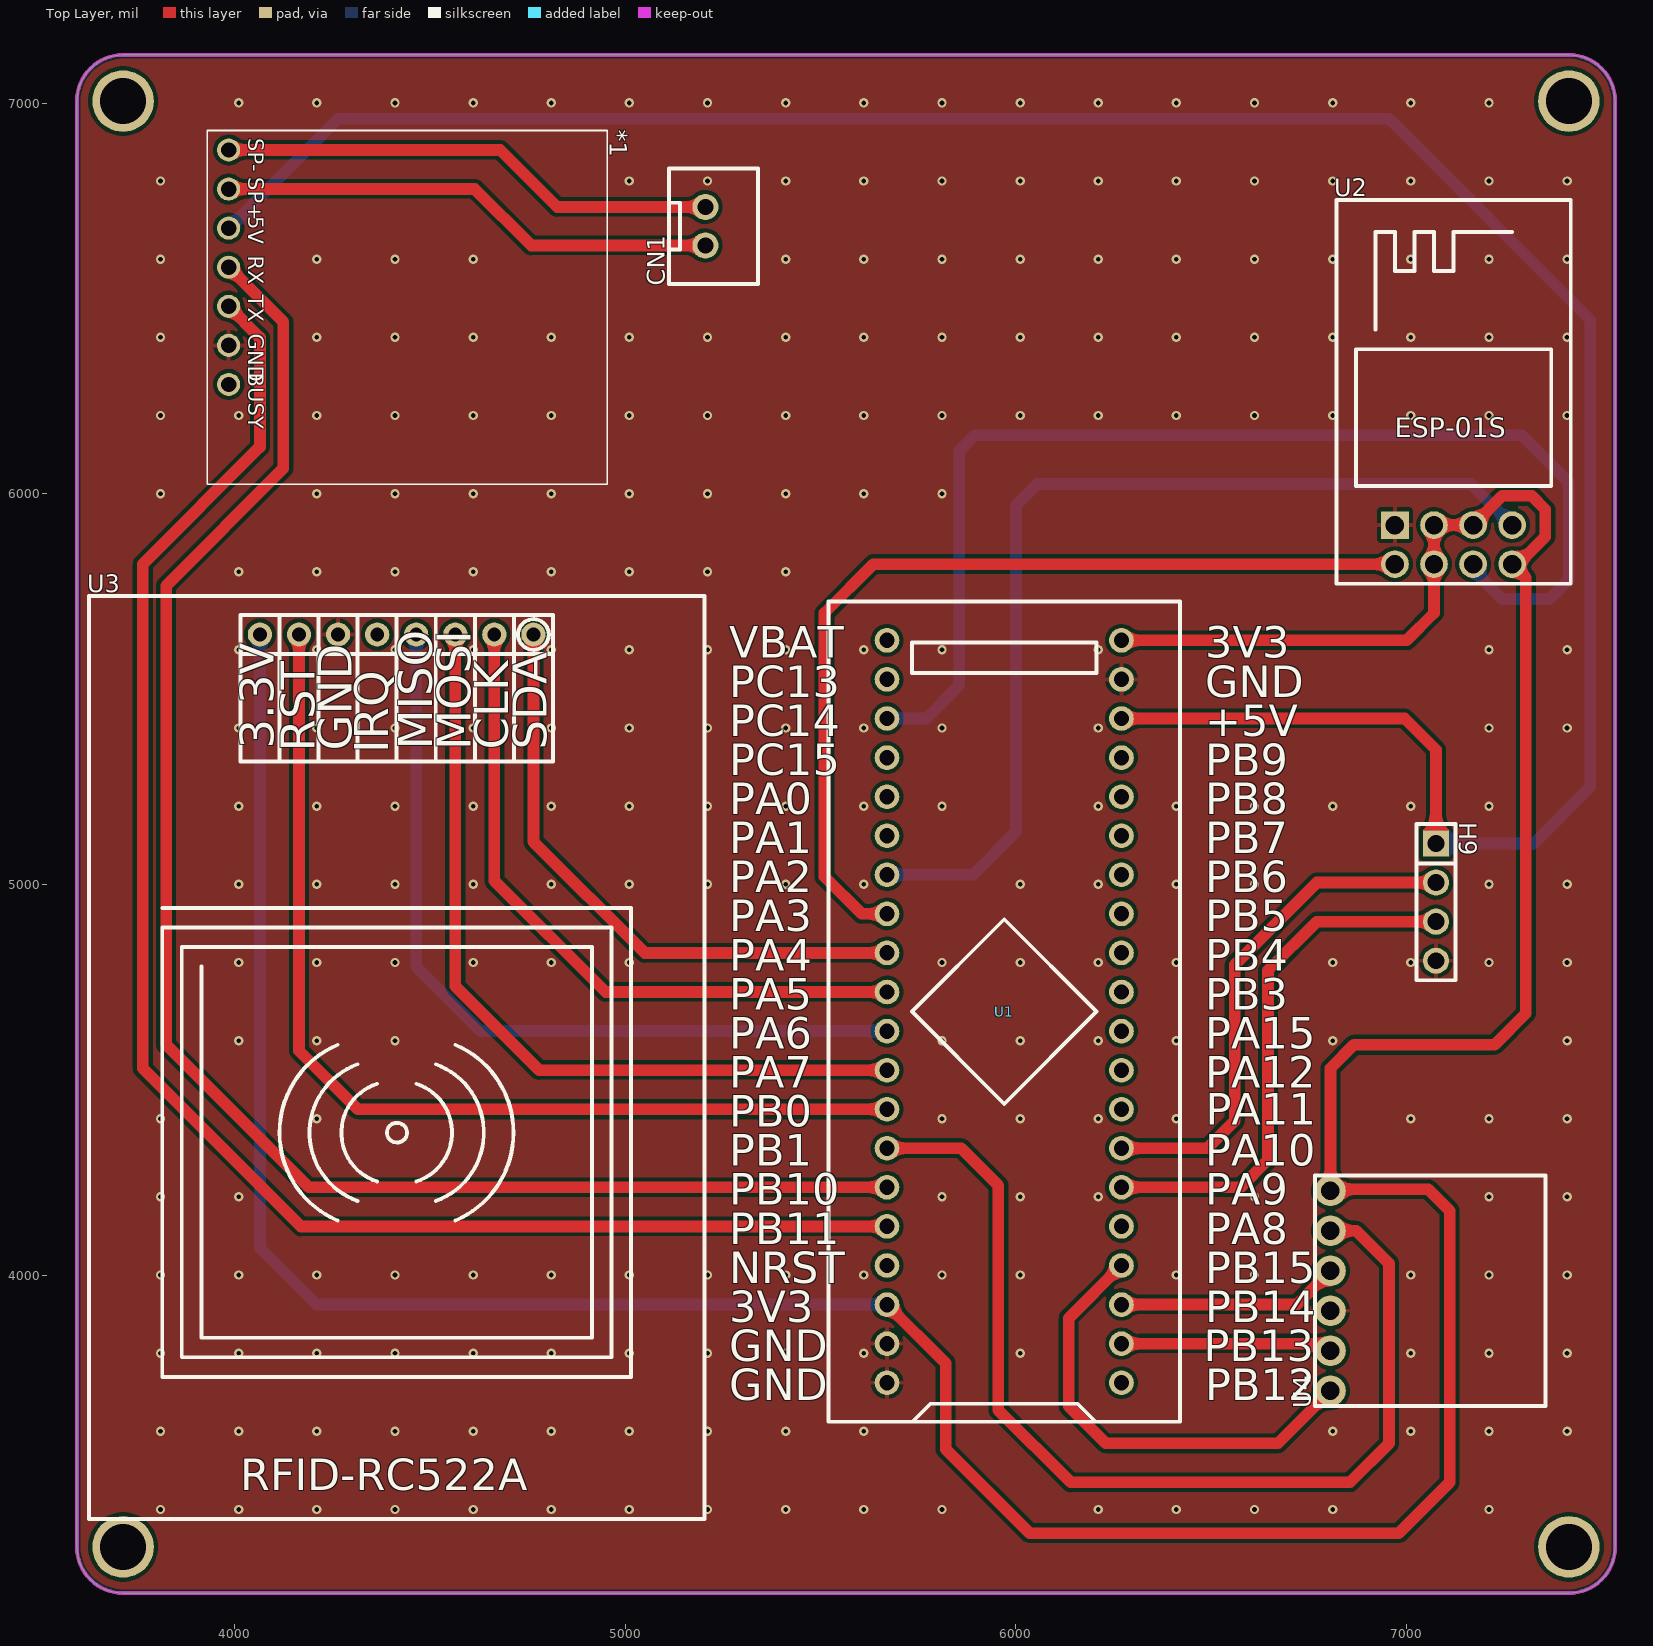
[diagram p0: Top Layer view]
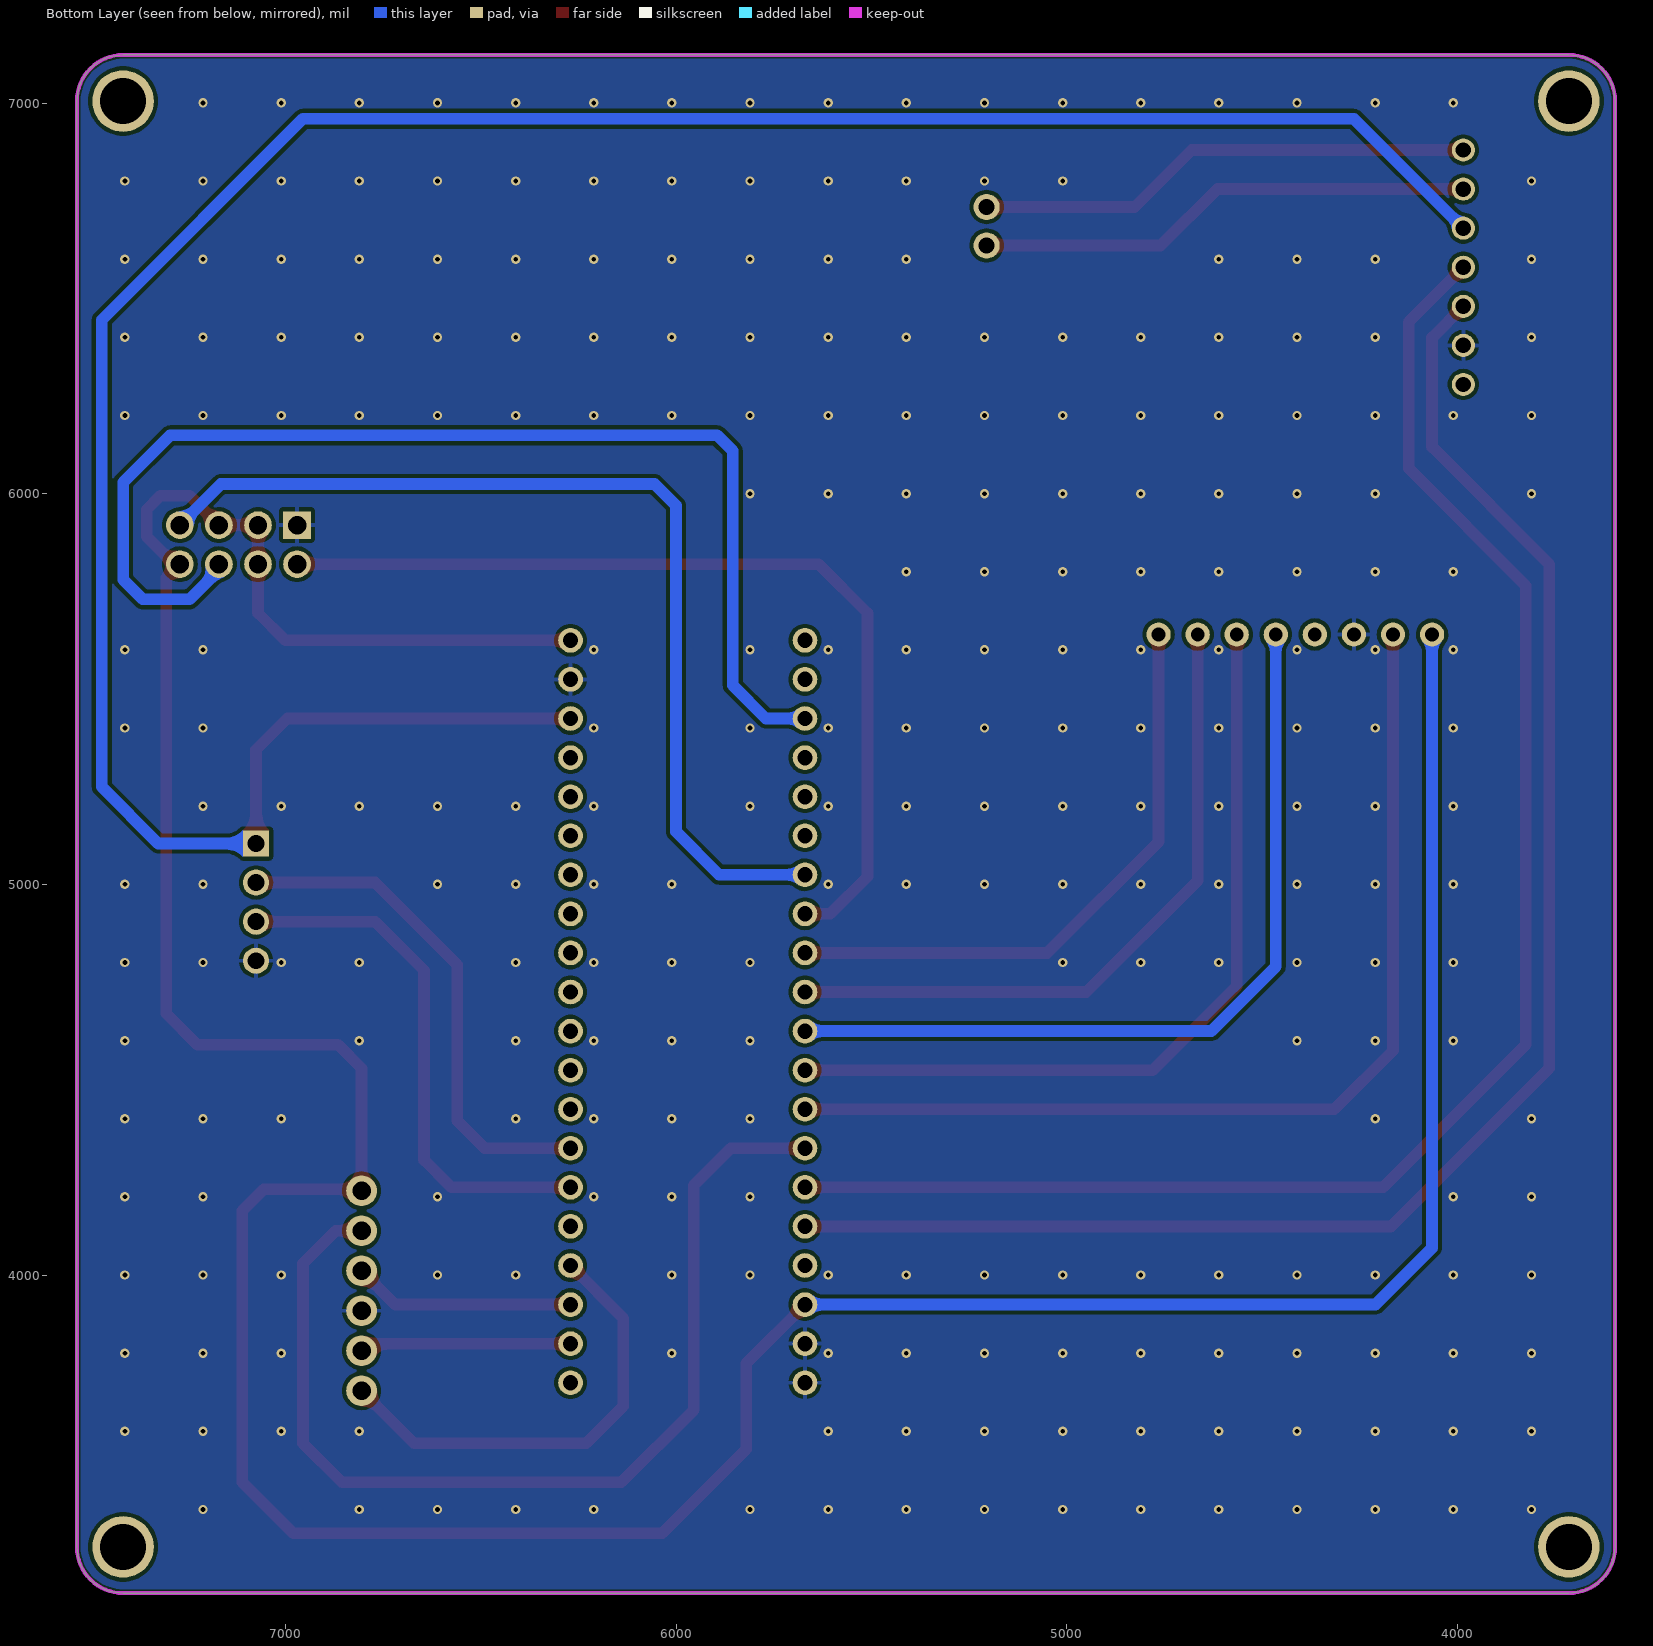
[diagram p1: Bottom Layer view, seen from below]
# Altium PCB MISC51107.pcbdoc
Units mil, origin at the board's own origin, x right, y up, seen from the top; angles counter-clockwise.
Board outline 3937.01 x 3937.01 mil, 2 copper layers (Top Layer, Bottom Layer), stack 62.206 mil thick; 7 components, 39 nets, 79 pads, 259 vias.

## Layer stack, top to bottom
Top Solder Mask Layer: solder mask 0.394, Dk 3.3
Top Layer: signal copper 1.379
Dielectric1: surface 59.449, FR4, Dk 4.5
Bottom Layer: signal copper 1.378
Bottom Solder Mask Layer: solder mask 0.394, Dk 3.3

## Board outline
3714.61,7123.5 ccw(c3714.61,7005.39) 3596.5,7005.39 3596.5,3304.61 ccw(c3714.61,3304.61) 3714.61,3186.5 7415.39,3186.5 ccw(c7415.39,3304.61) 7533.5,3304.61 7533.5,7005.39 ccw(c7415.39,7005.39) 7415.39,7123.5 3714.61,7123.5

## Design rules (kind name [scope] priority, off if disabled: settings)
BoardOutlineClearance copperThickness2oz_1 [All] p2 off: genericclearance=7.99 ignorepadtopadclearanceinfootprint=FALSE except(0: Arc-SplitContinuation Track-SplitContinuation SMDPad-SplitContinuation THPad-SplitContinuation Via-SplitContinuation Fill-SplitContinuation Region-SplitContinuation Poly-SplitContinuation Text-SplitContinuation Hole-SplitContinuation; 5.98: Arc-CutoutEdge Track-CutoutEdge SMDPad-CutoutEdge THPad-CutoutEdge Via-CutoutEdge Text-CutoutEdge; 6.9: Hole-OutlineEdge Hole-CutoutEdge; 10: Poly-OutlineEdge Poly-CutoutEdge; 11.81: Arc-OutlineEdge Track-OutlineEdge SMDPad-OutlineEdge THPad-OutlineEdge Via-OutlineEdge Fill-OutlineEdge Region-OutlineEdge Text-OutlineEdge Fill-CutoutEdge Region-CutoutEdge)
BoardOutlineClearance Plane_innerPlane_1 [All] p4 off: genericclearance=4.02 ignorepadtopadclearanceinfootprint=FALSE except(0: Arc-SplitContinuation Track-SplitContinuation SMDPad-SplitContinuation THPad-SplitContinuation Via-SplitContinuation Fill-SplitContinuation Region-SplitContinuation Poly-SplitContinuation Text-SplitContinuation Hole-SplitContinuation; 5.98: Arc-CutoutEdge Track-CutoutEdge SMDPad-CutoutEdge THPad-CutoutEdge Via-CutoutEdge Text-CutoutEdge; 6.9: Hole-OutlineEdge Hole-CutoutEdge; 10: Poly-OutlineEdge Poly-CutoutEdge; 11.81: Arc-OutlineEdge Track-OutlineEdge SMDPad-OutlineEdge THPad-OutlineEdge Via-OutlineEdge Fill-OutlineEdge Region-OutlineEdge Text-OutlineEdge Fill-CutoutEdge Region-CutoutEdge)
BoardOutlineClearance Copper_copperRegion_1 [All] p6 off: genericclearance=4.02 ignorepadtopadclearanceinfootprint=FALSE except(0: Arc-SplitContinuation Track-SplitContinuation SMDPad-SplitContinuation THPad-SplitContinuation Via-SplitContinuation Fill-SplitContinuation Region-SplitContinuation Poly-SplitContinuation Text-SplitContinuation Hole-SplitContinuation; 5.98: Arc-CutoutEdge Track-CutoutEdge SMDPad-CutoutEdge THPad-CutoutEdge Via-CutoutEdge Text-CutoutEdge; 6.9: Hole-OutlineEdge Hole-CutoutEdge; 10: Poly-OutlineEdge Poly-CutoutEdge; 11.81: Arc-OutlineEdge Track-OutlineEdge SMDPad-OutlineEdge THPad-OutlineEdge Via-OutlineEdge Fill-OutlineEdge Region-OutlineEdge Text-OutlineEdge Fill-CutoutEdge Region-CutoutEdge)
BoardOutlineClearance Copper_copperRegion_copperThickness1oz_1 [All] p8 off: genericclearance=4.02 ignorepadtopadclearanceinfootprint=FALSE except(0: Arc-SplitContinuation Track-SplitContinuation SMDPad-SplitContinuation THPad-SplitContinuation Via-SplitContinuation Fill-SplitContinuation Region-SplitContinuation Poly-SplitContinuation Text-SplitContinuation Hole-SplitContinuation; 5.98: Arc-CutoutEdge Track-CutoutEdge SMDPad-CutoutEdge THPad-CutoutEdge Via-CutoutEdge Text-CutoutEdge; 6.9: Hole-OutlineEdge Hole-CutoutEdge; 10: Poly-OutlineEdge Poly-CutoutEdge; 11.81: Arc-OutlineEdge Track-OutlineEdge SMDPad-OutlineEdge THPad-OutlineEdge Via-OutlineEdge Fill-OutlineEdge Region-OutlineEdge Text-OutlineEdge Fill-CutoutEdge Region-CutoutEdge)
BoardOutlineClearance Copper_copperRegion_Copper_copperRegion_1 [All] p10 off: genericclearance=4.02 ignorepadtopadclearanceinfootprint=FALSE except(0: Arc-SplitContinuation Track-SplitContinuation SMDPad-SplitContinuation THPad-SplitContinuation Via-SplitContinuation Fill-SplitContinuation Region-SplitContinuation Poly-SplitContinuation Text-SplitContinuation Hole-SplitContinuation; 5.98: Arc-CutoutEdge Track-CutoutEdge SMDPad-CutoutEdge THPad-CutoutEdge Via-CutoutEdge Text-CutoutEdge; 6.9: Hole-OutlineEdge Hole-CutoutEdge; 10: Poly-OutlineEdge Poly-CutoutEdge; 11.81: Arc-OutlineEdge Track-OutlineEdge SMDPad-OutlineEdge THPad-OutlineEdge Via-OutlineEdge Fill-OutlineEdge Region-OutlineEdge Text-OutlineEdge Fill-CutoutEdge Region-CutoutEdge)
BoardOutlineClearance copperThickness1oz_1 [All] p12: genericclearance=4.02 ignorepadtopadclearanceinfootprint=FALSE except(0: Arc-SplitContinuation Track-SplitContinuation SMDPad-SplitContinuation THPad-SplitContinuation Via-SplitContinuation Fill-SplitContinuation Region-SplitContinuation Poly-SplitContinuation Text-SplitContinuation Hole-SplitContinuation; 5.98: Arc-CutoutEdge Track-CutoutEdge SMDPad-CutoutEdge THPad-CutoutEdge Via-CutoutEdge Text-CutoutEdge; 6.9: Hole-OutlineEdge Hole-CutoutEdge; 10: Poly-OutlineEdge Poly-CutoutEdge; 11.81: Arc-OutlineEdge Track-OutlineEdge SMDPad-OutlineEdge THPad-OutlineEdge Via-OutlineEdge Fill-OutlineEdge Region-OutlineEdge Text-OutlineEdge Fill-CutoutEdge Region-CutoutEdge)
Clearance copperThickness2oz [All] p1 off: gap=7.99 ignorepadtopadclearanceinfootprint=FALSE except(5.98: SMDPad-Track SMDPad-SMDPad THPad-Track SMDPad-THPad THPad-THPad Track-Via SMDPad-Via THPad-Via Via-Via Fill-SMDPad Region-SMDPad Fill-THPad Region-THPad Fill-Via Region-Via Fill-Fill Fill-Region Region-Region Arc-Track Arc-SMDPad Arc-THPad Arc-Via Fill-Arc Region-Arc Arc-Arc Text-Track SMDPad-Text Text-THPad Text-Via Fill-Text Region-Text Arc-Text Text-Text; 6.9: Hole-Track Hole-SMDPad Hole-THPad Hole-Via Fill-Hole Region-Hole Hole-Arc Hole-Text; 10: Poly-Track Poly-SMDPad Poly-THPad Poly-Via Poly-Fill Poly-Region Poly-Poly Poly-Arc Poly-Text Poly-Hole; 11.81: Fill-Track Region-Track)
Clearance Plane_innerPlane [All] p3 off: gap=4.02 ignorepadtopadclearanceinfootprint=FALSE except(5.98: SMDPad-Track SMDPad-SMDPad THPad-Track SMDPad-THPad THPad-THPad Track-Via SMDPad-Via THPad-Via Via-Via Fill-SMDPad Region-SMDPad Fill-THPad Region-THPad Fill-Via Region-Via Fill-Fill Fill-Region Region-Region Arc-Track Arc-SMDPad Arc-THPad Arc-Via Fill-Arc Region-Arc Arc-Arc Text-Track SMDPad-Text Text-THPad Text-Via Fill-Text Region-Text Arc-Text Text-Text; 6.9: Hole-Track Hole-SMDPad Hole-THPad Hole-Via Fill-Hole Region-Hole Hole-Arc Hole-Text; 10: Poly-Track Poly-SMDPad Poly-THPad Poly-Via Poly-Fill Poly-Region Poly-Poly Poly-Arc Poly-Text Poly-Hole; 11.81: Fill-Track Region-Track)
Clearance Copper_copperRegion [All] p5 off: gap=4.02 ignorepadtopadclearanceinfootprint=FALSE except(5.98: SMDPad-Track SMDPad-SMDPad THPad-Track SMDPad-THPad THPad-THPad Track-Via SMDPad-Via THPad-Via Via-Via Fill-SMDPad Region-SMDPad Fill-THPad Region-THPad Fill-Via Region-Via Fill-Fill Fill-Region Region-Region Arc-Track Arc-SMDPad Arc-THPad Arc-Via Fill-Arc Region-Arc Arc-Arc Text-Track SMDPad-Text Text-THPad Text-Via Fill-Text Region-Text Arc-Text Text-Text; 6.9: Hole-Track Hole-SMDPad Hole-THPad Hole-Via Fill-Hole Region-Hole Hole-Arc Hole-Text; 10: Poly-Track Poly-SMDPad Poly-THPad Poly-Via Poly-Fill Poly-Region Poly-Poly Poly-Arc Poly-Text Poly-Hole; 11.81: Fill-Track Region-Track)
Clearance Copper_copperRegion_copperThickness1oz [All] p7 off: gap=4.02 ignorepadtopadclearanceinfootprint=FALSE except(5.98: SMDPad-Track SMDPad-SMDPad THPad-Track SMDPad-THPad THPad-THPad Track-Via SMDPad-Via THPad-Via Via-Via Fill-SMDPad Region-SMDPad Fill-THPad Region-THPad Fill-Via Region-Via Fill-Fill Fill-Region Region-Region Arc-Track Arc-SMDPad Arc-THPad Arc-Via Fill-Arc Region-Arc Arc-Arc Text-Track SMDPad-Text Text-THPad Text-Via Fill-Text Region-Text Arc-Text Text-Text; 6.9: Hole-Track Hole-SMDPad Hole-THPad Hole-Via Fill-Hole Region-Hole Hole-Arc Hole-Text; 10: Poly-Track Poly-SMDPad Poly-THPad Poly-Via Poly-Fill Poly-Region Poly-Poly Poly-Arc Poly-Text Poly-Hole; 11.81: Fill-Track Region-Track)
Clearance Copper_copperRegion_Copper_copperRegion [All] p9 off: gap=4.02 ignorepadtopadclearanceinfootprint=FALSE except(5.98: SMDPad-Track SMDPad-SMDPad THPad-Track SMDPad-THPad THPad-THPad Track-Via SMDPad-Via THPad-Via Via-Via Fill-SMDPad Region-SMDPad Fill-THPad Region-THPad Fill-Via Region-Via Fill-Fill Fill-Region Region-Region Arc-Track Arc-SMDPad Arc-THPad Arc-Via Fill-Arc Region-Arc Arc-Arc Text-Track SMDPad-Text Text-THPad Text-Via Fill-Text Region-Text Arc-Text Text-Text; 6.9: Hole-Track Hole-SMDPad Hole-THPad Hole-Via Fill-Hole Region-Hole Hole-Arc Hole-Text; 10: Poly-Track Poly-SMDPad Poly-THPad Poly-Via Poly-Fill Poly-Region Poly-Poly Poly-Arc Poly-Text Poly-Hole; 11.81: Fill-Track Region-Track)
Clearance copperThickness1oz [All] p11: gap=4.02 ignorepadtopadclearanceinfootprint=FALSE except(5.98: SMDPad-Track SMDPad-SMDPad THPad-Track SMDPad-THPad THPad-THPad Track-Via SMDPad-Via THPad-Via Via-Via Fill-SMDPad Region-SMDPad Fill-THPad Region-THPad Fill-Via Region-Via Fill-Fill Fill-Region Region-Region Arc-Track Arc-SMDPad Arc-THPad Arc-Via Fill-Arc Region-Arc Arc-Arc Text-Track SMDPad-Text Text-THPad Text-Via Fill-Text Region-Text Arc-Text Text-Text; 6.9: Hole-Track Hole-SMDPad Hole-THPad Hole-Via Fill-Hole Region-Hole Hole-Arc Hole-Text; 10: Poly-Track Poly-SMDPad Poly-THPad Poly-Via Poly-Fill Poly-Region Poly-Poly Poly-Arc Poly-Text Poly-Hole; 11.81: Fill-Track Region-Track)
DiffPairsRouting differentialPair [All] p1: maxlimit=6 minlimit=6 mostfreqgap=6 toplayer_minwidth=5 toplayer_prefwidth=10 toplayer_maxwidth=100 toplayer_mingap=6 toplayer_prefgap=6 toplayer_maxgap=6 bottomlayer_minwidth=5 bottomlayer_prefwidth=10 bottomlayer_maxwidth=100 bottomlayer_mingap=6 bottomlayer_prefgap=6 bottomlayer_maxgap=6 maxuncoupledlength=10
HoleToHoleClearance otherClearance [All] p1: gap=11.81 allowstackedmicrovias=TRUE
Length netLength [All] p1: minlimit=0 maxlimit=0
PasteMaskExpansion pasteMaskExpansion [All] p1: expansion=0
PlaneConnect innerPlane [All] p1: planeconnectstyle=Relief reliefexpansion=20 reliefentries=4 reliefconductorwidth=10 reliefairgap=10
PolygonConnect copperRegion_copperThickness1oz [All] p1 off: connectstyle=Relief reliefconductorwidth=10 reliefentries=4 polygonreliefangle="90 Angle" airgapwidth=10 via.connectstyle=Relief via.reliefconductorwidth=10 via.reliefentries=4 via.polygonreliefangle="90 Angle" via.airgapwidth=10
PolygonConnect copperRegion_Copper_copperRegion [All] p2 off: connectstyle=Relief reliefconductorwidth=10 reliefentries=4 polygonreliefangle="90 Angle" airgapwidth=10 via.connectstyle=Relief via.reliefconductorwidth=10 via.reliefentries=4 via.polygonreliefangle="90 Angle" via.airgapwidth=10
PolygonConnect copperRegion [All] p3: connectstyle=Relief reliefconductorwidth=10 reliefentries=4 polygonreliefangle="90 Angle" airgapwidth=10 via.connectstyle=Relief via.reliefconductorwidth=10 via.reliefentries=4 via.polygonreliefangle="90 Angle" via.airgapwidth=10
RoutingVias viaSize [All] p1: holewidth=12.01 width=24.02 viastyle="Through Hole" minholewidth=11.81 minwidth=19.68 maxholewidth=248.03 maxwidth=393.7
SolderMaskExpansion solderMaskExpansion [IsVia] p1: expansion=-1000 istentingtop=TRUE
SolderMaskExpansion solderMaskExpansion [All] p2: expansion=2 istentingtop=FALSE
Width copperThickness2oz_2 [All] p1 off: maxlimit=100 minlimit=8 preferedwidth=10
Width copperThickness1oz_2 [All] p2: maxlimit=100 minlimit=5 preferedwidth=10

## Components (designator, comment, footprint, x,y, rotation, side; value= is the part's Value field where it differs from the comment)
*1 "LU6288" LU6288 3985,6880 r270 top
CN1 "XH2.54*2P_直插" CONN-TH_2P-P2.50-XH2.54-2P 5205,6685 r90 top
H9 "" HDR-TH_4P-P2.54-V-M 7075,4955 r270 top
U1 "STM32F103C8T6-Card" CONN-TH_L53.3-W22.9_STM32F103C8T6-CARD 5970,4675 r90 top
U2 "ESP-01S" WIFIM-TH_ESP-01S 7120,5870 r0 top
U3 "" RC522 4165,5640 r0 top
U4 "" W25Q64 6765,3665 r90 top

## Footprints (in the part's own frame and the unit in brackets; to place one, negate y for a bottom-side part, rotate by r counter-clockwise, add the part's x,y. Pads: shape width x height; smd on the part's side, far side on the other; paste and mask are expansions set on the pad)
CONN-TH_2P-P2.50-XH2.54-2P [mm]
  round 1.7 hole 1.05 paste+0 mask+0.05: 1(1.25,0) 2(-1.25,0)
  silkscreen extent -3.75,-3.42 3.75,2.37
CONN-TH_L53.3-W22.9_STM32F103C8T6-CARD [mm]
  round 1.6 hole 1: 1(-24.13,-7.62) 2(-21.59,-7.62) 3(-19.05,-7.62) 4(-16.51,-7.62) 5(-13.97,-7.62) 6(-11.43,-7.62) 7(-8.89,-7.62) 8(-6.35,-7.62) 9(-3.81,-7.62) 10(-1.27,-7.62) 11(1.27,-7.62) 12(3.81,-7.62) 13(6.35,-7.62) 14(8.89,-7.62) 15(11.43,-7.62) 16(13.97,-7.62) 17(16.51,-7.62) 18(19.05,-7.62) 19(21.59,-7.62) 20(24.13,-7.62) 21(24.13,7.62) 22(21.59,7.62) 23(19.05,7.62) 24(16.51,7.62) 25(13.97,7.62) 26(11.43,7.62) 27(8.89,7.62) 28(6.35,7.62) 29(3.81,7.62) 30(1.27,7.62) 31(-1.27,7.62) 32(-3.81,7.62) 33(-6.35,7.62) 34(-8.89,7.62) 35(-11.43,7.62) 36(-13.97,7.62) 37(-16.51,7.62) 38(-19.05,7.62) 39(-21.59,7.62) 40(-24.13,7.62)
  silkscreen extent -26.67,-11.43 26.67,11.43
HDR-TH_4P-P2.54-V-M [mm]
  rect 1.7x1.7 hole 1.1: 1(-3.81,0)
  round 1.7 hole 1.1: 2(-1.27,0) 3(1.27,0) 4(3.81,0)
  silkscreen extent -5.08,-1.27 5.08,1.27
LU6288 [mm]
  round 1.5 hole 1: 1(0,0) 2(2.54,0) 3(5.08,0) 4(7.62,0) 5(10.16,0) 6(12.7,0) 7(15.24,0)
  silkscreen extent -1.27,-1.4 21.73,24.6
RC522 [mm]
  round 1.575 hole 0.889 paste+0 mask+0.102: 1(-2.54,0) 2(0,0) 3(2.54,0) 4(5.08,0) 5(7.62,0) 6(10.16,0) 7(12.7,0) 8(15.24,0)
  silkscreen extent -13.65,-57.5 26.35,2.5
W25Q64 [mm]
  round 2 hole 1.2: 1(1,-1.016) 2(3.6,-1.016) 3(6.2,-1.016) 4(8.8,-1.016) 5(11.4,-1.016) 6(14,-1.016)
  silkscreen extent 0,-15 15,0
WIFIM-TH_ESP-01S [mm]
  rect 1.8x1.8 hole 1.2: 1(-3.81,1.27)
  round 1.8 hole 1.2: 2(-1.27,1.27) 3(1.27,1.27) 4(3.81,1.27) 5(3.81,-1.27) 6(1.27,-1.27) 7(-1.27,-1.27) 8(-3.81,-1.27)
  silkscreen extent -7.62,-2.54 7.62,22.4

## Free pads (board coordinates)
  round 157.48 hole 118.11: 1(3714.61,7005.39) 1(3714.61,3304.61) 1(7415.39,7005.39) 1(7415.39,3304.61)

## Via types
v1: diameter 24.02, hole 12, Top Layer to Bottom Layer, 259 vias

## Nets (pads, with @x,y where several pads share a name; then routed paths per layer and width w, separated by ;. In a path a pad name is that pad's centre, name@x,y a point inside that pad or via, vN(x,y) a via of type N, cw(c..) or ccw(c..) an arc to the next point about the centre after c; other vN are vias at no path point)
$1N17261: *1.2 CN1.2 | length 1279.7
  Top Layer w30: *1.2 4615,6780 4759.22,6635.78 CN1.2
$1N17262: *1.1 CN1.1 | length 1280.4
  Top Layer w30: *1.1 4680,6880 4825.78,6734.22 CN1.1
+5V: *1.3 H9.1 U1.18 | length 6542.5
  Top Layer w30: U1.18 6995,5425 7075,5345 H9.1
  Bottom Layer w30: *1.3 4265,6960 6955,6960 7470,6445 7470,5250 7325,5105 H9.1
GND: *1.6 H9.4 U1.19 U1.39 U1.40 U2.1 U3.3 U4.3
  other v1: 3810.6,3400.6 4010.6,3400.6 4210.6,3400.6 4410.6,3400.6 4610.6,3400.6 4810.6,3400.6 5010.6,3400.6 5210.6,3400.6 5410.6,3400.6 5610.6,3400.6 5810.6,3400.6 6210.6,3400.6 6410.6,3400.6 6610.6,3400.6 6810.6,3400.6 7210.6,3400.6 3810.6,3600.6 4010.6,3600.6 4210.6,3600.6 4410.6,3600.6 4610.6,3600.6 4810.6,3600.6 5010.6,3600.6 5210.6,3600.6 5410.6,3600.6 5610.6,3600.6 6810.6,3600.6 7010.6,3600.6 7210.6,3600.6 7410.6,3600.6 3810.6,3800.6 4010.6,3800.6 4210.6,3800.6 4410.6,3800.6 4610.6,3800.6 4810.6,3800.6 5010.6,3800.6 5210.6,3800.6 5410.6,3800.6 5610.6,3800.6 6010.6,3800.6 7010.6,3800.6 7210.6,3800.6 7410.6,3800.6 3810.6,4000.6 4010.6,4000.6 4210.6,4000.6 4410.6,4000.6 4610.6,4000.6 4810.6,4000.6 5010.6,4000.6 5210.6,4000.6 5410.6,4000.6 5610.6,4000.6 5810.6,4000.6 6010.6,4000.6 6410.6,4000.6 6610.6,4000.6 7010.6,4000.6 7210.6,4000.6 7410.6,4000.6 3810.6,4200.6 4010.6,4200.6 5810.6,4200.6 6010.6,4200.6 6210.6,4200.6 6610.6,4200.6 7210.6,4200.6 7410.6,4200.6 3810.6,4400.6 4210.6,4400.6 5810.6,4400.6 6010.6,4400.6 6210.6,4400.6 6410.6,4400.6 7010.6,4400.6 7210.6,4400.6 7410.6,4400.6 4010.6,4600.6 4210.6,4600.6 4410.6,4600.6 5810.6,4600.6 6010.6,4600.6 6210.6,4600.6 6410.6,4600.6 6810.6,4600.6 7410.6,4600.6 4010.6,4800.6 4210.6,4800.6 4410.6,4800.6 4610.6,4800.6 4810.6,4800.6 5010.6,4800.6 5810.6,4800.6 6010.6,4800.6 6210.6,4800.6 6410.6,4800.6 6810.6,4800.6 7010.6,4800.6 7210.6,4800.6 7410.6,4800.6 4010.6,5000.6 4210.6,5000.6 4410.6,5000.6 4610.6,5000.6 4810.6,5000.6 5010.6,5000.6 5210.6,5000.6 5410.6,5000.6 5610.6,5000.6 6010.6,5000.6 6210.6,5000.6 6410.6,5000.6 6610.6,5000.6 7210.6,5000.6 7410.6,5000.6 4010.6,5200.6 4210.6,5200.6 4410.6,5200.6 4610.6,5200.6 4810.6,5200.6 5010.6,5200.6 5210.6,5200.6 5410.6,5200.6 5610.6,5200.6 5810.6,5200.6 6210.6,5200.6 6410.6,5200.6 6610.6,5200.6 6810.6,5200.6 7010.6,5200.6 7210.6,5200.6 4010.6,5400.6 4210.6,5400.6 4410.6,5400.6 4610.6,5400.6 4810.6,5400.6 5010.6,5400.6 5210.6,5400.6 5410.6,5400.6 5610.6,5400.6 5810.6,5400.6 6210.6,5400.6 7210.6,5400.6 7410.6,5400.6 4010.6,5600.6 4210.6,5600.6 4410.6,5600.6 4610.6,5600.6 4810.6,5600.6 5010.6,5600.6 5210.6,5600.6 5410.6,5600.6 5610.6,5600.6 5810.6,5600.6 6210.6,5600.6 7210.6,5600.6 7410.6,5600.6 4010.6,5800.6 4210.6,5800.6 4410.6,5800.6 4610.6,5800.6 4810.6,5800.6 5010.6,5800.6 5210.6,5800.6 5410.6,5800.6 3810.6,6000.6 4210.6,6000.6 4410.6,6000.6 4610.6,6000.6 4810.6,6000.6 5010.6,6000.6 5210.6,6000.6 5410.6,6000.6 5610.6,6000.6 5810.6,6000.6 3810.6,6200.6 4010.6,6200.6 4210.6,6200.6 4410.6,6200.6 4610.6,6200.6 4810.6,6200.6 5010.6,6200.6 5210.6,6200.6 5410.6,6200.6 5610.6,6200.6 5810.6,6200.6 6010.6,6200.6 6210.6,6200.6 6410.6,6200.6 6610.6,6200.6 6810.6,6200.6 7010.6,6200.6 7210.6,6200.6 7410.6,6200.6 3810.6,6400.6 4210.6,6400.6 4410.6,6400.6 4610.6,6400.6 4810.6,6400.6 5010.6,6400.6 5210.6,6400.6 5410.6,6400.6 5610.6,6400.6 5810.6,6400.6 6010.6,6400.6 6210.6,6400.6 6410.6,6400.6 6610.6,6400.6 6810.6,6400.6 7010.6,6400.6 7210.6,6400.6 7410.6,6400.6 3810.6,6600.6 4210.6,6600.6 4410.6,6600.6 4610.6,6600.6 5410.6,6600.6 5610.6,6600.6 5810.6,6600.6 6010.6,6600.6 6210.6,6600.6 6410.6,6600.6 6610.6,6600.6 6810.6,6600.6 7010.6,6600.6 7210.6,6600.6 7410.6,6600.6 3810.6,6800.6 5010.6,6800.6 5210.6,6800.6 5410.6,6800.6 5610.6,6800.6 5810.6,6800.6 6010.6,6800.6 6210.6,6800.6 6410.6,6800.6 6610.6,6800.6 6810.6,6800.6 7010.6,6800.6 7210.6,6800.6 7410.6,6800.6 4010.6,7000.6 4210.6,7000.6 4410.6,7000.6 4610.6,7000.6 4810.6,7000.6 5010.6,7000.6 5210.6,7000.6 5410.6,7000.6 5610.6,7000.6 5810.6,7000.6 6010.6,7000.6 6210.6,7000.6 6410.6,7000.6 6610.6,7000.6 6810.6,7000.6 7010.6,7000.6 7210.6,7000.6
NRST: U1.37
PA0: U1.25
PA1: U1.26
PA2: U1.27 U2.4 | length 2546.8
  Bottom Layer w30: U1.27 5890,5025 6000,5135 6000,5970 6055,6025 7165,6025 U2.4
PA3: U1.28 U2.8 | length 2386.1
  Top Layer w30: U1.28 5605,4925 5510,5020 5510,5695 5635,5820 U2.8
PA4: U1.29 U3.8 | length 1553
  Top Layer w30: U3.8 4765,5110 5050,4825 U1.29
PA5: U1.30 U3.7 | length 1753
  Top Layer w30: U3.7 4665,5010 4950,4725 U1.30
PA6: U1.31 U3.5 | length 2123.3
  Bottom Layer w30: U3.5 4465,4790 4630,4625 U1.31
PA7: U1.32 U3.6 | length 2094.1
  Top Layer w30: U3.6 4565,4740 4780,4525 U1.32
PA8: U1.5
PA9: H9.3 U1.6 | length 1370.8
  Top Layer w30: U1.6 6575,4225 6645,4295 6645,4780 6770,4905 H9.3
PA10: H9.2 U1.7 | length 1321
  Top Layer w30: U1.7 6490,4325 6560,4395 6560,4795 6770,5005 H9.2
PA11: U1.8
PA12: U1.9
PA15: U1.10
PB0: U1.33 U3.2 | length 2632.1
  Top Layer w30: U3.2 4165,4575 4315,4425 U1.33
PB1: U1.34 U4.5 | length 2662.1
  Top Layer w30: U1.34 5860,4325 5955,4230 5955,3655 6140,3470 6855,3470 6955,3570 6955,4030 6871.18,4113.82 U4.5
PB3: U1.11
PB4: U1.12
PB5: U1.13
PB6: U1.14
PB7: U1.15
PB8: U1.16
PB9: U1.17
PB10: *1.4 U1.35 | length 4168.4
  Top Layer w30: *1.4 4125,6440 4125,6065 3825,5765 3825,4590 4190,4225 U1.35
PB11: *1.5 U1.36 | length 4180.2
  Top Layer w30: *1.5 4065,6400 4065,6120 3765,5820 3765,4530 4170,4125 U1.36
PB12: U1.1
PB13: U1.2 U4.2 | length 542.6
  Top Layer w30: U1.2 6786.73,3825 U4.2
PB14: U1.3 U4.4 | length 570.8
  Top Layer w30: U1.3 6718.55,3925 U4.4
PB15: U1.4 U4.1 | length 1180.9
  Top Layer w30: U1.4 6135,3890 6135,3665 6230,3570 6670.63,3570 U4.1
PC13: U1.22
PC14: U1.23 U2.6 | length 3008.3
  Bottom Layer w30: U1.23 5770,5425 5855,5510 5855,6110 5895,6150 7295,6150 7415,6030 7415,5780 7365,5730 7245,5730 7170,5805 U2.6
PC15: U1.24
VBAT: U1.21
VCC: U1.20 U1.38 U2.2 U2.3 U2.5 U2.7 U3.1 U4.6 | length 9729.3
  Top Layer w30: U1.38 5820,3775 5820,3555 6035,3340 6980,3340 7110,3470 7110,4165 7055,4220 6808.82,4220 U4.6 6805,4530 6865,4590 7225,4590 7305,4670 7305,5785 U2.5 7285,5820 7355,5890 7355,5960 7320,5995 7245,5995 U2.3 U2.2 U2.7 7070,5695 7000,5625 U1.20
  Bottom Layer w30: U3.1 4065,4070 4210,3925 U1.38
pads on no net: *1.7 U3.4

## Polygon pours and split planes (outlines as drawn)
GND on Bottom Layer (solid, remove dead copper, pour order 2): 3525,7245 3525,3080 7700,3080 7700,7245
GND on Top Layer (solid, remove dead copper, pour order 2): 3000,7415 3000,3000 7930,3000 7930,7415

## Keep-outs
Board Outline Layer:
  the board outline again, w10

## Other copper
Top Layer:
  region net PB13: 6312.88,3840 6312.88,3810 6310.37,3809.81 6307.53,3809.26 6304.5,3808.41 6301.39,3807.31 6298.34,3806 6295.48,3804.55 6292.93,3802.99 6290.83,3801.38 6290.83,3848.62 6292.93,3847.02 6295.48,3845.46 6298.34,3844 6301.39,3842.7 6304.5,3841.59 6307.53,3840.74 6310.37,3840.2
  region net PB14: 6312.88,3940 6312.88,3910 6310.37,3909.81 6307.53,3909.26 6304.5,3908.41 6301.39,3907.31 6298.34,3906 6295.48,3904.55 6292.93,3902.99 6290.83,3901.38 6290.83,3948.62 6292.93,3947.02 6295.48,3945.46 6298.34,3944 6301.39,3942.7 6304.5,3941.59 6307.53,3940.74 6310.37,3940.2
  region net PB15: 6250.28,3984.07 6229.07,4005.29 6230.71,4007.2 6232.33,4009.59 6233.87,4012.34 6235.29,4015.32 6236.53,4018.4 6237.52,4021.45 6238.22,4024.35 6238.56,4026.97 6271.97,3993.57 6269.35,3993.22 6266.45,3992.52 6263.4,3991.53 6260.32,3990.3 6257.34,3988.88 6254.59,3987.33 6252.2,3985.71
  region net PA9: 6312.88,4240 6312.88,4210 6310.37,4209.81 6307.53,4209.26 6304.5,4208.41 6301.39,4207.31 6298.34,4206 6295.48,4204.55 6292.93,4202.99 6290.83,4201.38 6290.83,4248.62 6292.93,4247.02 6295.48,4245.46 6298.34,4244 6301.39,4242.7 6304.5,4241.59 6307.53,4240.74 6310.37,4240.2
  region net PA10: 6312.88,4340 6312.88,4310 6310.37,4309.81 6307.53,4309.26 6304.5,4308.41 6301.39,4307.31 6298.34,4306 6295.48,4304.55 6292.93,4302.99 6290.83,4301.38 6290.83,4348.62 6292.93,4347.02 6295.48,4345.46 6298.34,4344 6301.39,4342.7 6304.5,4341.59 6307.53,4340.74 6310.37,4340.2
  region net +5V: 6312.88,5440 6312.88,5410 6310.37,5409.81 6307.53,5409.26 6304.5,5408.41 6301.39,5407.31 6298.34,5406 6295.48,5404.55 6292.93,5402.99 6290.83,5401.38 6290.83,5448.62 6292.93,5447.02 6295.48,5445.46 6298.34,5444 6301.39,5442.7 6304.5,5441.59 6307.53,5440.74 6310.37,5440.2
  region net VCC: 6312.88,5640 6312.88,5610 6310.37,5609.81 6307.53,5609.26 6304.5,5608.41 6301.39,5607.31 6298.34,5606 6295.48,5604.55 6292.93,5602.99 6290.83,5601.38 6290.83,5648.62 6292.93,5647.02 6295.48,5645.46 6298.34,5644 6301.39,5642.7 6304.5,5641.59 6307.53,5640.74 6310.37,5640.2
  region net PA3: 5627.12,4910 5627.12,4940 5629.63,4940.2 5632.47,4940.74 5635.5,4941.59 5638.61,4942.7 5641.66,4944 5644.52,4945.46 5647.07,4947.02 5649.17,4948.62 5649.17,4901.38 5647.07,4902.99 5644.52,4904.55 5641.66,4906 5638.61,4907.31 5635.5,4908.41 5632.47,4909.26 5629.63,4909.81
  region net PA4: 5627.12,4810 5627.12,4840 5629.63,4840.2 5632.47,4840.74 5635.5,4841.59 5638.61,4842.7 5641.66,4844 5644.52,4845.46 5647.07,4847.02 5649.17,4848.62 5649.17,4801.38 5647.07,4802.99 5644.52,4804.55 5641.66,4806 5638.61,4807.31 5635.5,4808.41 5632.47,4809.26 5629.63,4809.81
  region net PA5: 5627.12,4710 5627.12,4740 5629.63,4740.2 5632.47,4740.74 5635.5,4741.59 5638.61,4742.7 5641.66,4744 5644.52,4745.46 5647.07,4747.02 5649.17,4748.62 5649.17,4701.38 5647.07,4702.99 5644.52,4704.55 5641.66,4706 5638.61,4707.31 5635.5,4708.41 5632.47,4709.26 5629.63,4709.81
  region net PA7: 5627.12,4510 5627.12,4540 5629.63,4540.2 5632.47,4540.74 5635.5,4541.59 5638.61,4542.7 5641.66,4544 5644.52,4545.46 5647.07,4547.02 5649.17,4548.62 5649.17,4501.38 5647.07,4502.99 5644.52,4504.55 5641.66,4506 5638.61,4507.31 5635.5,4508.41 5632.47,4509.26 5629.63,4509.81
  region net PB0: 5627.12,4410 5627.12,4440 5629.63,4440.2 5632.47,4440.74 5635.5,4441.59 5638.61,4442.7 5641.66,4444 5644.52,4445.46 5647.07,4447.02 5649.17,4448.62 5649.17,4401.38 5647.07,4402.99 5644.52,4404.55 5641.66,4406 5638.61,4407.31 5635.5,4408.41 5632.47,4409.26 5629.63,4409.81
  region net PB1: 5712.88,4340 5712.88,4310 5710.37,4309.81 5707.53,4309.26 5704.5,4308.41 5701.39,4307.31 5698.34,4306 5695.48,4304.55 5692.93,4302.99 5690.83,4301.38 5690.83,4348.62 5692.93,4347.02 5695.48,4345.46 5698.34,4344 5701.39,4342.7 5704.5,4341.59 5707.53,4340.74 5710.37,4340.2
  region net PB10: 5627.12,4210 5627.12,4240 5629.63,4240.2 5632.47,4240.74 5635.5,4241.59 5638.61,4242.7 5641.66,4244 5644.52,4245.46 5647.07,4247.02 5649.17,4248.62 5649.17,4201.38 5647.07,4202.99 5644.52,4204.55 5641.66,4206 5638.61,4207.31 5635.5,4208.41 5632.47,4209.26 5629.63,4209.81
  region net PB11: 5627.12,4110 5627.12,4140 5629.63,4140.2 5632.47,4140.74 5635.5,4141.59 5638.61,4142.7 5641.66,4144 5644.52,4145.46 5647.07,4147.02 5649.17,4148.62 5649.17,4101.38 5647.07,4102.99 5644.52,4104.55 5641.66,4106 5638.61,4107.31 5635.5,4108.41 5632.47,4109.26 5629.63,4109.81
  region net VCC: 5710.93,3905.29 5689.71,3884.07 5687.8,3885.71 5685.41,3887.33 5682.66,3888.88 5679.68,3890.3 5676.6,3891.53 5673.55,3892.52 5670.65,3893.22 5668.03,3893.57 5701.43,3926.97 5701.78,3924.35 5702.48,3921.45 5703.47,3918.4 5704.71,3915.32 5706.12,3912.34 5707.67,3909.59 5709.29,3907.2
  region net $1N17262: 4025.2,6895 4025.2,6865 4022.67,6864.84 4019.89,6864.39 4016.97,6863.68 4014.03,6862.77 4011.19,6861.69 4008.59,6860.48 4006.32,6859.19 4004.53,6857.85 4004.53,6902.15 4006.32,6900.81 4008.59,6899.52 4011.19,6898.31 4014.03,6897.23 4016.97,6896.32 4019.89,6895.61 4022.67,6895.16
  region net $1N17261: 4025.2,6795 4025.2,6765 4022.67,6764.84 4019.89,6764.39 4016.97,6763.68 4014.03,6762.77 4011.19,6761.69 4008.59,6760.48 4006.32,6759.19 4004.53,6757.85 4004.53,6802.15 4006.32,6800.81 4008.59,6799.52 4011.19,6798.31 4014.03,6797.23 4016.97,6796.32 4019.89,6795.61 4022.67,6795.16
  region net PB11: 4024.03,6462.18 4002.82,6440.97 4000.92,6442.64 3998.63,6444.29 3996.06,6445.86 3993.34,6447.29 3990.57,6448.53 3987.87,6449.52 3985.36,6450.2 3983.15,6450.53 4014.47,6481.85 4014.8,6479.64 4015.48,6477.13 4016.47,6474.43 4017.71,6471.66 4019.14,6468.94 4020.71,6466.37 4022.36,6464.08
  region net PB10: 4024.03,6562.18 4002.82,6540.97 4000.92,6542.64 3998.63,6544.29 3996.06,6545.86 3993.34,6547.29 3990.57,6548.53 3987.87,6549.52 3985.36,6550.2 3983.15,6550.53 4014.47,6581.85 4014.8,6579.64 4015.48,6577.13 4016.47,6574.43 4017.71,6571.66 4019.14,6568.94 4020.71,6566.37 4022.36,6564.08
  region net $1N17261: 5159.44,6620.78 5159.44,6650.78 5161.93,6651.01 5164.82,6651.65 5167.97,6652.65 5171.25,6653.94 5174.52,6655.47 5177.63,6657.18 5180.46,6659 5182.87,6660.88 5182.87,6610.69 5180.46,6612.57 5177.63,6614.39 5174.52,6616.1 5171.25,6617.63 5167.97,6618.92 5164.82,6619.92 5161.93,6620.56
  region net $1N17262: 5159.44,6719.22 5159.44,6749.22 5161.93,6749.44 5164.82,6750.08 5167.97,6751.08 5171.25,6752.37 5174.52,6753.9 5177.63,6755.61 5180.46,6757.43 5182.87,6759.31 5182.87,6709.12 5180.46,6711 5177.63,6712.82 5174.52,6714.53 5171.25,6716.06 5167.97,6717.35 5164.82,6718.35 5161.93,6718.99
  region net +5V: 7060,5183.46 7090,5183.46 7090.4,5176.35 7091.58,5169.33 7093.54,5162.48 7096.24,5155.89 7099.66,5149.64 7103.75,5143.81 7108.46,5138.46 7041.54,5138.46 7046.25,5143.81 7050.34,5149.64 7053.76,5155.89 7056.46,5162.48 7058.42,5169.33 7059.6,5176.35 7060,5183.46
  region net PA10: 7029.44,4990 7029.44,5020 7031.93,5020.23 7034.82,5020.87 7037.97,5021.86 7041.25,5023.16 7044.52,5024.68 7047.63,5026.39 7050.46,5028.21 7052.87,5030.1 7052.87,4979.9 7050.46,4981.79 7047.63,4983.61 7044.52,4985.32 7041.25,4986.84 7037.97,4988.14 7034.82,4989.13 7031.93,4989.77
  region net PA9: 7029.44,4890 7029.44,4920 7031.93,4920.23 7034.82,4920.87 7037.97,4921.86 7041.25,4923.16 7044.52,4924.68 7047.63,4926.39 7050.46,4928.21 7052.87,4930.1 7052.87,4879.9 7050.46,4881.79 7047.63,4883.61 7044.52,4885.32 7041.25,4886.84 7037.97,4888.14 7034.82,4889.13 7031.93,4889.77
  region net VCC: 7085,5871.76 7055,5871.76 7054.74,5874.23 7054.01,5877.18 7052.86,5880.44 7051.38,5883.89 7049.63,5887.37 7047.68,5890.74 7045.58,5893.85 7043.43,5896.56 7096.57,5896.56 7094.42,5893.85 7092.32,5890.74 7090.37,5887.37 7088.62,5883.89 7087.14,5880.44 7085.99,5877.18 7085.26,5874.23
  region net VCC: 7118.24,5935 7118.24,5905 7115.77,5904.74 7112.82,5904.01 7109.56,5902.86 7106.11,5901.38 7102.63,5899.63 7099.26,5897.68 7096.15,5895.58 7093.44,5893.43 7093.44,5946.57 7096.15,5944.42 7099.26,5942.32 7102.63,5940.37 7106.11,5938.62 7109.56,5937.14 7112.82,5935.99 7115.77,5935.26
  region net VCC: 7121.76,5905 7121.76,5935 7124.23,5935.26 7127.18,5935.99 7130.44,5937.14 7133.89,5938.62 7137.37,5940.37 7140.74,5942.32 7143.85,5944.42 7146.56,5946.57 7146.56,5893.43 7143.85,5895.58 7140.74,5897.68 7137.37,5899.63 7133.89,5901.38 7130.44,5902.86 7127.18,5904.01 7124.23,5904.74
  region net VCC: 7193.5,5964.72 7214.72,5943.5 7213.15,5941.57 7211.59,5938.97 7210.09,5935.85 7208.7,5932.37 7207.48,5928.67 7206.48,5924.9 7205.75,5921.22 7205.36,5917.78 7167.78,5955.36 7171.22,5955.75 7174.9,5956.48 7178.67,5957.48 7182.37,5958.7 7185.85,5960.09 7188.97,5961.59 7191.57,5963.15
  region net VCC: 7314.72,5796.5 7293.5,5775.28 7291.57,5776.85 7288.97,5778.41 7285.85,5779.91 7282.37,5781.3 7278.67,5782.52 7274.9,5783.52 7271.22,5784.25 7267.78,5784.64 7305.36,5822.22 7305.75,5818.78 7306.48,5815.1 7307.48,5811.33 7308.7,5807.63 7310.09,5804.15 7311.59,5801.03 7313.15,5798.43
  region net VCC: 7305.87,5862.08 7315.83,5829.62 7314.43,5828 7312.83,5825.79 7309.3,5820.1 7305.85,5813.58 7304.34,5810.35 7303.08,5807.3 7278.47,5854.41 7281.68,5853.94 7285.28,5853.97 7289.09,5854.45 7292.97,5855.34 7296.74,5856.6 7300.26,5858.17 7303.36,5860.01
  region net VCC: 7085,5771.76 7055,5771.76 7054.74,5774.23 7054.01,5777.18 7052.86,5780.44 7051.38,5783.89 7049.63,5787.37 7047.68,5790.74 7045.58,5793.85 7043.43,5796.56 7096.57,5796.56 7094.42,5793.85 7092.32,5790.74 7090.37,5787.37 7088.62,5783.89 7087.14,5780.44 7085.99,5777.18 7085.26,5774.23
  region net VCC: 7055,5868.24 7085,5868.24 7085.26,5865.77 7085.99,5862.82 7087.14,5859.56 7088.62,5856.11 7090.37,5852.63 7092.32,5849.26 7094.42,5846.15 7096.57,5843.44 7043.43,5843.44 7045.58,5846.15 7047.68,5849.26 7049.63,5852.63 7051.38,5856.11 7052.86,5859.56 7054.01,5862.82 7054.74,5865.77
  region net PA3: 6921.76,5805 6921.76,5835 6924.23,5835.26 6927.18,5835.99 6930.44,5837.14 6933.89,5838.62 6937.37,5840.37 6940.74,5842.32 6943.85,5844.42 6946.56,5846.57 6946.56,5793.43 6943.85,5795.58 6940.74,5797.68 6937.37,5799.63 6933.89,5801.38 6930.44,5802.86 6927.18,5804.01 6924.23,5804.74
  region net PA4: 4780,5597.79 4750,5597.79 4749.81,5600.3 4749.29,5603.13 4748.48,5606.14 4747.42,5609.2 4746.17,5612.2 4744.78,5615 4743.29,5617.47 4741.75,5619.49 4788.25,5619.49 4786.71,5617.47 4785.22,5615 4783.83,5612.2 4782.58,5609.2 4781.52,5606.14 4780.71,5603.13 4780.19,5600.3
  region net PA5: 4680,5597.79 4650,5597.79 4649.81,5600.3 4649.29,5603.13 4648.48,5606.14 4647.42,5609.2 4646.17,5612.2 4644.78,5615 4643.29,5617.47 4641.75,5619.49 4688.25,5619.49 4686.71,5617.47 4685.22,5615 4683.83,5612.2 4682.58,5609.2 4681.52,5606.14 4680.71,5603.13 4680.19,5600.3
  region net PA7: 4580,5597.79 4550,5597.79 4549.81,5600.3 4549.29,5603.13 4548.48,5606.14 4547.42,5609.2 4546.17,5612.2 4544.78,5615 4543.29,5617.47 4541.75,5619.49 4588.25,5619.49 4586.71,5617.47 4585.22,5615 4583.83,5612.2 4582.58,5609.2 4581.52,5606.14 4580.71,5603.13 4580.19,5600.3
  region net PB0: 4180,5597.79 4150,5597.79 4149.81,5600.3 4149.29,5603.13 4148.48,5606.14 4147.42,5609.2 4146.17,5612.2 4144.78,5615 4143.29,5617.47 4141.75,5619.49 4188.25,5619.49 4186.71,5617.47 4185.22,5615 4183.83,5612.2 4182.58,5609.2 4181.52,5606.14 4180.71,5603.13 4180.19,5600.3
  region net PB15: 6777.71,3655.86 6756.49,3677.08 6757.99,3679.03 6759.49,3681.84 6760.95,3685.32 6762.31,3689.32 6763.52,3693.64 6764.53,3698.11 6765.27,3702.57 6765.71,3706.84 6807.47,3665.08 6803.2,3664.64 6798.74,3663.9 6794.27,3662.89 6789.95,3661.68 6785.95,3660.32 6782.47,3658.86 6779.66,3657.36
  region net PB13: 6740.67,3810 6768.08,3840 6772.49,3840.43 6779.41,3841.56 6787.56,3843.15 6795.64,3844.97 6768.23,3792.66 6767.49,3794.28 6766.52,3795.9 6765.35,3797.48 6764,3799.03 6760.81,3801.96 6757.13,3804.58 6753.11,3806.8 6748.92,3808.51 6746.82,3809.14 6744.72,3809.61 6742.67,3809.9
  region net PB14: 6777.71,3962.95 6756.49,3984.16 6757.99,3986.12 6759.49,3988.92 6760.95,3992.41 6762.31,3996.4 6763.52,4000.72 6764.53,4005.2 6765.27,4009.66 6765.71,4013.92 6807.47,3972.16 6803.2,3971.73 6798.74,3970.99 6794.27,3969.98 6789.95,3968.77 6785.95,3967.41 6782.47,3965.95 6779.66,3964.44
  region net PB1: 6858.6,4128.82 6858.6,4098.82 6856.16,4098.49 6853.11,4097.57 6849.62,4096.14 6845.83,4094.28 6841.92,4092.08 6838.04,4089.63 6834.36,4087 6831.04,4084.29 6831.04,4143.35 6834.36,4140.64 6838.04,4138.01 6841.92,4135.56 6845.83,4133.36 6849.62,4131.5 6853.11,4130.07 6856.16,4129.15
  region net VCC: 6790,4269.78 6820,4269.78 6820.33,4267.34 6821.25,4264.29 6822.68,4260.8 6824.54,4257.01 6826.74,4253.1 6829.19,4249.22 6831.82,4245.54 6834.53,4242.22 6775.47,4242.22 6778.18,4245.54 6780.81,4249.22 6783.26,4253.1 6785.46,4257.01 6787.32,4260.8 6788.75,4264.29 6789.67,4267.34
  region net VCC: 6855.61,4235 6861.34,4205 6860.05,4204.91 6858.6,4204.65 6855.34,4203.65 6851.71,4202.11 6847.88,4200.1 6844.01,4197.73 6840.27,4195.08 6836.8,4192.24 6833.78,4189.32 6828.05,4248.1 6831.65,4245.65 6835.52,4243.29 6839.51,4241.07 6843.46,4239.09 6847.21,4237.42 6850.59,4236.13 6853.45,4235.29
Bottom Layer:
  region net PC14: 5712.88,5440 5712.88,5410 5710.37,5409.81 5707.53,5409.26 5704.5,5408.41 5701.39,5407.31 5698.34,5406 5695.48,5404.55 5692.93,5402.99 5690.83,5401.38 5690.83,5448.62 5692.93,5447.02 5695.48,5445.46 5698.34,5444 5701.39,5442.7 5704.5,5441.59 5707.53,5440.74 5710.37,5440.2
  region net PA2: 5712.88,5040 5712.88,5010 5710.37,5009.81 5707.53,5009.26 5704.5,5008.41 5701.39,5007.31 5698.34,5006 5695.48,5004.55 5692.93,5002.99 5690.83,5001.38 5690.83,5048.62 5692.93,5047.02 5695.48,5045.46 5698.34,5044 5701.39,5042.7 5704.5,5041.59 5707.53,5040.74 5710.37,5040.2
  region net PA6: 5627.12,4610 5627.12,4640 5629.63,4640.2 5632.47,4640.74 5635.5,4641.59 5638.61,4642.7 5641.66,4644 5644.52,4645.46 5647.07,4647.02 5649.17,4648.62 5649.17,4601.38 5647.07,4602.99 5644.52,4604.55 5641.66,4606 5638.61,4607.31 5635.5,4608.41 5632.47,4609.26 5629.63,4609.81
  region net VCC: 5627.12,3910 5627.12,3940 5629.63,3940.2 5632.47,3940.74 5635.5,3941.59 5638.61,3942.7 5641.66,3944 5644.52,3945.46 5647.07,3947.02 5649.17,3948.62 5649.17,3901.38 5647.07,3902.99 5644.52,3904.55 5641.66,3906 5638.61,3907.31 5635.5,3908.41 5632.47,3909.26 5629.63,3909.81
  region net +5V: 4002.82,6719.03 4024.03,6697.82 4022.36,6695.92 4020.71,6693.63 4019.14,6691.06 4017.71,6688.34 4016.47,6685.57 4015.48,6682.87 4014.8,6680.36 4014.47,6678.15 3983.15,6709.47 3985.36,6709.8 3987.87,6710.48 3990.57,6711.47 3993.34,6712.71 3996.06,6714.14 3998.63,6715.71 4000.92,6717.36
  region net +5V: 7153.46,5120 7153.46,5090 7146.35,5089.6 7139.33,5088.42 7132.48,5086.46 7125.89,5083.76 7119.64,5080.34 7113.81,5076.25 7108.46,5071.54 7108.46,5138.46 7113.81,5133.75 7119.64,5129.66 7125.89,5126.24 7132.48,5123.54 7139.33,5121.58 7146.35,5120.4 7153.46,5120
  region net PA2: 7225.28,5943.5 7246.5,5964.72 7248.43,5963.15 7251.03,5961.59 7254.15,5960.09 7257.63,5958.7 7261.33,5957.48 7265.1,5956.48 7268.78,5955.75 7272.22,5955.36 7234.64,5917.78 7234.25,5921.22 7233.52,5924.9 7232.52,5928.67 7231.3,5932.37 7229.91,5935.85 7228.41,5938.97 7226.85,5941.57
  region net PC14: 7212.08,5784.13 7179.62,5774.17 7178,5775.57 7175.79,5777.17 7170.1,5780.7 7163.58,5784.15 7160.35,5785.66 7157.3,5786.92 7204.41,5811.53 7203.94,5808.32 7203.97,5804.72 7204.45,5800.91 7205.34,5797.03 7206.6,5793.26 7208.17,5789.74 7210.01,5786.64
  region net PA6: 4480,5597.79 4450,5597.79 4449.81,5600.3 4449.29,5603.13 4448.48,5606.14 4447.42,5609.2 4446.17,5612.2 4444.78,5615 4443.29,5617.47 4441.75,5619.49 4488.25,5619.49 4486.71,5617.47 4485.22,5615 4483.83,5612.2 4482.58,5609.2 4481.52,5606.14 4480.71,5603.13 4480.19,5600.3
  region net VCC: 4080,5597.79 4050,5597.79 4049.81,5600.3 4049.29,5603.13 4048.48,5606.14 4047.42,5609.2 4046.17,5612.2 4044.78,5615 4043.29,5617.47 4041.75,5619.49 4088.25,5619.49 4086.71,5617.47 4085.22,5615 4083.83,5612.2 4082.58,5609.2 4081.52,5606.14 4080.71,5603.13 4080.19,5600.3

## Silkscreen, mask and mechanical layers (free items; w line width, h text height)
Top Silkscreen Layer:
  text "VBAT" at 5265.95,5580 h80
  text "3V3" at 6484.16,5580 h80
  text "PC13" at 5265.95,5480 h80
  text "GND" at 6484.16,5480 h80
  text "PC14" at 5265.95,5380 h80
  text "+5V" at 6484.16,5380 h80
  text "PC15" at 5265.95,5280 h80
  text "PB9" at 6484.16,5280 h80
  text "PA0" at 5265.95,5180 h80
  text "PB8" at 6484.16,5180 h80
  text "PA1" at 5265.95,5080 h80
  text "PB7" at 6484.16,5080 h80
  text "PA2" at 5265.95,4980 h80
  text "PB6" at 6484.16,4980 h80
  text "PA3" at 5265.95,4880 h80
  text "PB5" at 6484.16,4880 h80
  text "PA4" at 5265.95,4780 h80
  text "PB4" at 6484.16,4780 h80
  text "PA5" at 5265.95,4680 h80
  text "PB3" at 6484.16,4680 h80
  text "PA6" at 5265.95,4580 h80
  text "PA15" at 6484.16,4580 h80
  text "PA7" at 5265.95,4480 h80
  text "PA12" at 6484.16,4480 h80
  text "PA11" at 6485.95,4385 h80
  text "PB0" at 5265.95,4380 h80
  text "PB1" at 5265.95,4280 h80
  text "PA10" at 6484.16,4280 h80
  text "PB10" at 5265.95,4180 h80
  text "PA9" at 6484.16,4180 h80
  text "PB11" at 5265.95,4080 h80
  text "PA8" at 6484.16,4080 h80
  text "NRST" at 5265.95,3980 h80
  text "PB15" at 6484.16,3980 h80
  text "3V3" at 5265.95,3880 h80
  text "PB14" at 6484.16,3880 h80
  text "GND" at 5265.95,3780 h80
  text "PB13" at 6480.95,3780 h80
  text "GND" at 5265.95,3680 h80
  text "PB12" at 6484.16,3680 h80